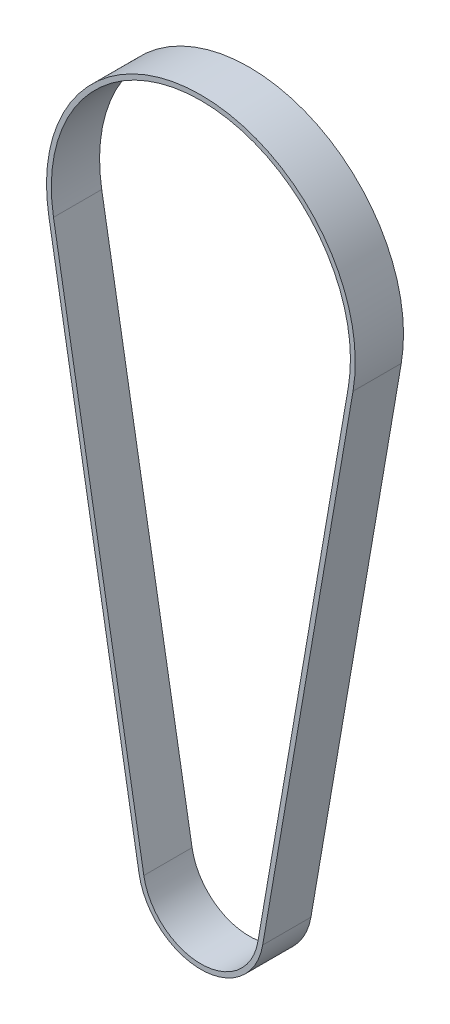
from build123d import *

# Parameters (mm, degrees)
EXTRUDE_1_DEPTH = 20


with BuildPart() as part:
    # 草图1 → 拉伸-薄壁1 (new body)
    with BuildSketch(Plane.XY):
        with BuildLine():
            Line((25.623145777, -228.410714286), (63.072358835, -10.857142857))
            ThreePointArc((63.072358835, -10.857142857), (0, 64), (-63.072358835, -10.857142857))
            Line((-63.072358835, -10.857142857), (-25.623145777, -228.410714286))
            ThreePointArc((-25.623145777, -228.410714286), (0, -250), (25.623145777, -228.410714286))
        make_face()
        with BuildLine():
            Line((23.652134563, -228.071428571), (61.101347621, -10.517857143))
            ThreePointArc((61.101347621, -10.517857143), (0, 62), (-61.101347621, -10.517857143))
            Line((-61.101347621, -10.517857143), (-23.652134563, -228.071428571))
            ThreePointArc((-23.652134563, -228.071428571), (0, -248), (23.652134563, -228.071428571))
        make_face(mode=Mode.SUBTRACT)
    extrude(amount=EXTRUDE_1_DEPTH)


solid = part.part
